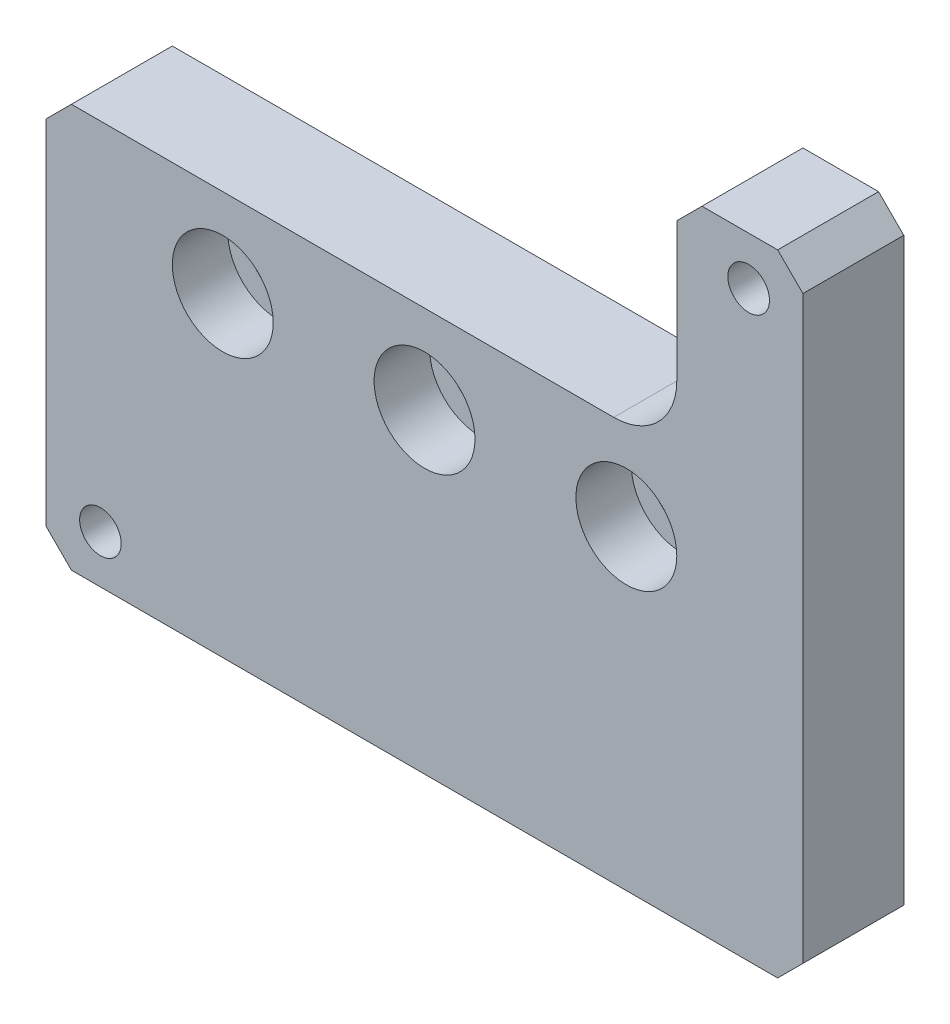
from build123d import *

# Parameters (mm, degrees)
SKETCH1_W                                           = 60
SKETCH1_H                                           = 50
BOSS_EXTRUDE1_DEPTH                                 = 8
CBORE_FOR_M4_HEX_SOCKET_HEAD_CAP_SCREW1_D           = 4.5
CBORE_FOR_M4_HEX_SOCKET_HEAD_CAP_SCREW1_CBORE_D     = 8
CBORE_FOR_M4_HEX_SOCKET_HEAD_CAP_SCREW1_CBORE_DEPTH = 4.4
M4_TAPPED_HOLE1_D                                   = 3.3
CHAMFER1_SIZE                                       = 2
SKETCH6_W                                           = 50
SKETCH6_H                                           = 18
CUT_EXTRUDE1_DEPTH                                  = 79.511145706
CHAMFER2_SIZE                                       = 2
FILLET1_R                                           = 5


with BuildPart() as part:
    # Sketch1 → Boss-Extrude1 (new body)
    with BuildSketch(Plane.XY):
        with Locations((30, 25)):
            Rectangle(SKETCH1_W, SKETCH1_H)
    extrude(amount=BOSS_EXTRUDE1_DEPTH)

    # CBORE for M4 Hex Socket Head Cap Screw1 (through all)
    with Locations(Plane.XY.offset(8)):
        with Locations((46, 25), (30, 25), (14, 25)):
            CounterBoreHole(CBORE_FOR_M4_HEX_SOCKET_HEAD_CAP_SCREW1_D / 2, CBORE_FOR_M4_HEX_SOCKET_HEAD_CAP_SCREW1_CBORE_D / 2, CBORE_FOR_M4_HEX_SOCKET_HEAD_CAP_SCREW1_CBORE_DEPTH)

    # M4 Tapped Hole1 (through all)
    with Locations(Plane.XY.offset(8)):
        with Locations((55.7, 46.2), (4.3, 3.8)):
            Hole(M4_TAPPED_HOLE1_D / 2)

    # Chamfer1
    chamfer1_edges = [part.edges().sort_by_distance(p)[0] for p in [
        (0, 50, 4),
        (60, 50, 4),
        (60, 0, 4),
        (0, 0, 4),
    ]]
    chamfer(chamfer1_edges, length=CHAMFER1_SIZE)

    # Sketch6 → Cut-Extrude1 (cut, through all)
    with BuildSketch(Plane(origin=(0, 0, 0), x_dir=(-1, 0, 0), z_dir=(0, 0, -1))):
        with Locations((-25, 41)):
            Rectangle(SKETCH6_W, SKETCH6_H)
    extrude(amount=-CUT_EXTRUDE1_DEPTH, mode=Mode.SUBTRACT)

    # Chamfer2
    chamfer2_edges = [part.edges().sort_by_distance(p)[0] for p in [
        (50, 50, 4),
        (0, 32, 4),
    ]]
    chamfer(chamfer2_edges, length=CHAMFER2_SIZE)

    # Fillet1
    fillet1_edges = [part.edges().sort_by_distance(p)[0] for p in [
        (50, 32, 4),
    ]]
    fillet(fillet1_edges, radius=FILLET1_R)


solid = part.part
